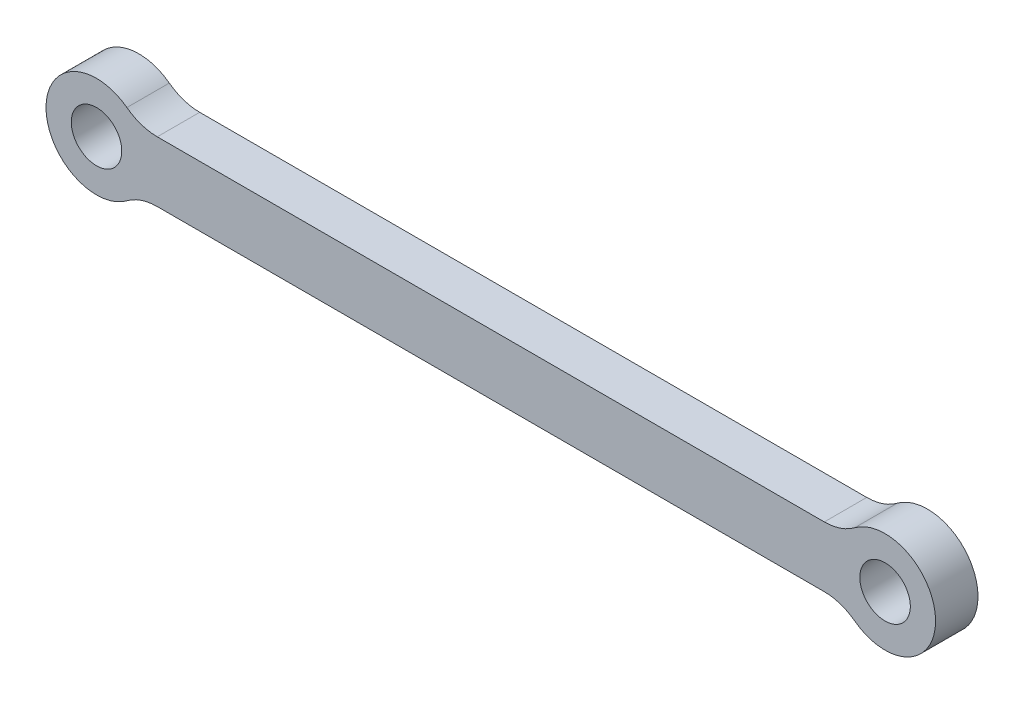
from build123d import *

# Parameters (mm, degrees)
SKETCH1_R           = 50
BOSS_EXTRUDE1_DEPTH = 84


with BuildPart() as part:
    # Sketch1 → Boss-Extrude1 (new body)
    with BuildSketch(Plane.XY):
        with BuildLine():
            Line((-617.326495153, 59.809220037), (703.165599022, 59.809220037))
            ThreePointArc((703.165599022, 59.809220037), (734.86369832, 64.966031031), (763.292575479, 79.904610019))
            ThreePointArc((763.292575479, 79.904610019), (923.419551935, 0), (763.292575479, -79.904610019))
            ThreePointArc((763.292575479, -79.904610019), (734.86369832, -64.966031031), (703.165599022, -59.809220037))
            Line((703.165599022, -59.809220037), (-617.326495153, -59.809220037))
            ThreePointArc((-617.326495153, -59.809220037), (-649.02459445, -64.966031031), (-677.453471609, -79.904610019))
            ThreePointArc((-677.453471609, -79.904610019), (-837.580448065, 0), (-677.453471609, 79.904610019))
            ThreePointArc((-677.453471609, 79.904610019), (-649.02459445, 64.966031031), (-617.326495153, 59.809220037))
        make_face()
        with Locations(Location((-737.580448065, 0, 0), (0, 0, 180))):
            Circle(SKETCH1_R, mode=Mode.SUBTRACT)
        with Locations(Location((823.419551935, 0, 0), (0, 0, 180))):
            Circle(SKETCH1_R, mode=Mode.SUBTRACT)
    extrude(amount=BOSS_EXTRUDE1_DEPTH)


solid = part.part
